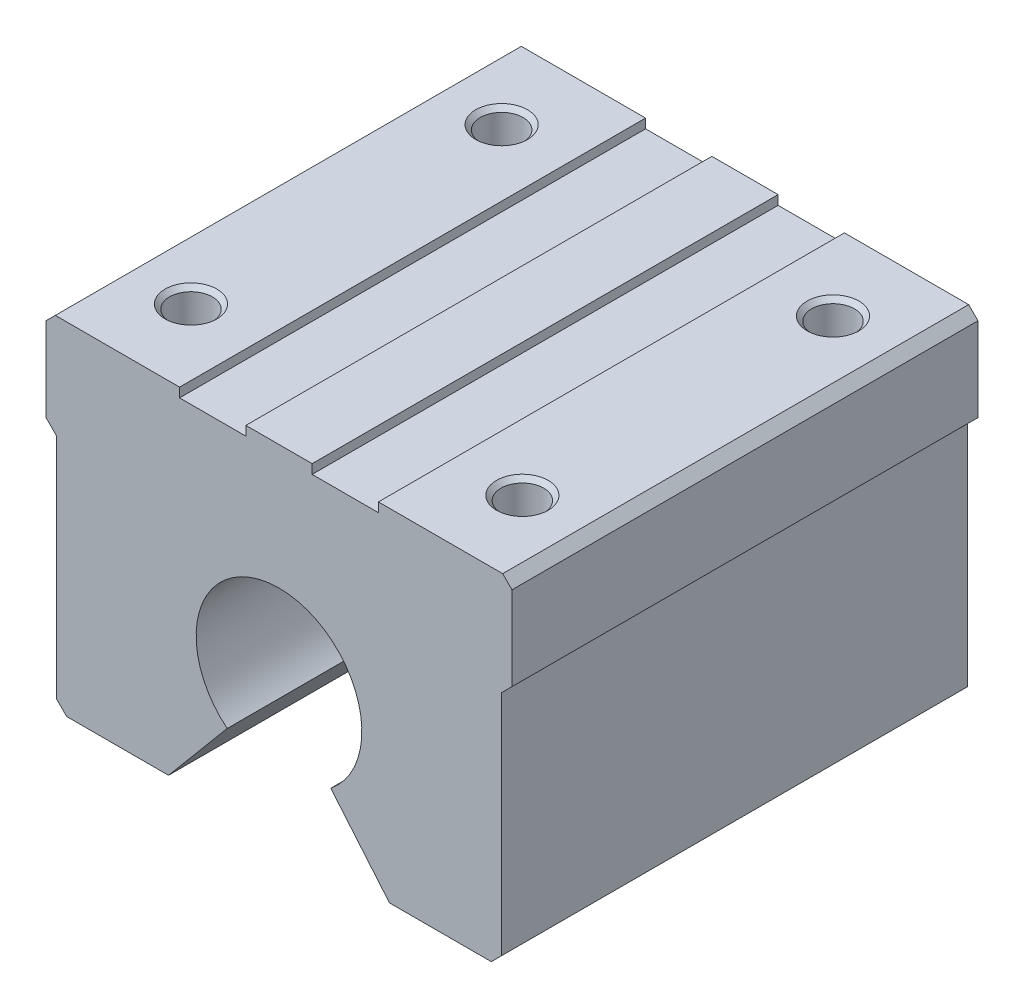
from build123d import *

# Parameters (mm, degrees)
SKETCH_1_W               = 45
SKETCH_1_H               = 45
EXTRUDE_1_DEPTH          = 33
SKETCH_2_W               = 6.4
SKETCH_2_H               = 0.9
CUT_EXTRUDE_1_DEPTH      = 68.5
SKETCH_3_W               = 6.4
SKETCH_3_H               = 0.9
CUT_EXTRUDE_2_DEPTH      = 68.5
SKETCH_4_W               = 1
SKETCH_4_H               = 24
CUT_EXTRUDE_3_DEPTH      = 68.5
CUT_EXTRUDE_4_DEPTH      = 68.5
SKETCH_6_W               = 1
SKETCH_6_H               = 24
CUT_EXTRUDE_5_DEPTH      = 68.500000167
DRAFT_1_ANGLE            = 45
DRAFT_2_ANGLE            = 45
DRAFT_3_ANGLE            = 40
HOLE_WIZARD_16_0_16_1_D  = 16.000000007
HOLE_WIZARD_M3_5_1_D     = 4.134
HOLE_WIZARD_M3_5_1_DEPTH = 15.60662
HOLE_WIZARD_M3_5_1_TIP   = 1.193383006
CHAMFER_1_SIZE           = 0.433
CHAMFER_2_SIZE           = 1
CHAMFER_3_SIZE           = 0.9
CUT_EXTRUDE_6_DEPTH      = 106.297198595


with BuildPart() as part:
    # 草图1 → 凸台-拉伸1 (new body)
    with BuildSketch(Plane.XZ.offset(-12)):
        with Locations((0, 230)):
            Rectangle(SKETCH_1_W, SKETCH_1_H)
    extrude(amount=-EXTRUDE_1_DEPTH)

    # 草图2 → 切除-拉伸1 (cut, through all)
    with BuildSketch(Plane.XY.offset(252.5)):
        with Locations((-6.4, 44.55)):
            Rectangle(SKETCH_2_W, SKETCH_2_H)
    extrude(amount=-CUT_EXTRUDE_1_DEPTH, mode=Mode.SUBTRACT)

    # 草图3 → 切除-拉伸2 (cut, through all)
    with BuildSketch(Plane.XY.offset(252.5)):
        with Locations((6.4, 44.55)):
            Rectangle(SKETCH_3_W, SKETCH_3_H)
    extrude(amount=-CUT_EXTRUDE_2_DEPTH, mode=Mode.SUBTRACT)

    # 草图4 → 切除-拉伸3 (cut, through all)
    with BuildSketch(Plane.XY.offset(252.5)):
        with Locations((22, 24)):
            Rectangle(SKETCH_4_W, SKETCH_4_H)
    extrude(amount=-CUT_EXTRUDE_3_DEPTH, mode=Mode.SUBTRACT)

    # 草图5 → 切除-拉伸4 (cut, through all)
    with BuildSketch(Plane.XY.offset(252.5)):
        with BuildLine():
            Line((-10.668119688, 12), (10.668119688, 12))
            add(Edge.make_bspline(
                [(5, 18.755002002), (6.889373229, 16.503334668), (8.778746459, 14.251667334), (10.668119688, 12)],
                knots=[0, 0, 0, 0, 1, 1, 1, 1], degree=3))
            Line((5, 18.755002002), (-10.668119688, 37.427539929))
            Line((-10.668119688, 37.427539929), (-10.668119688, 12))
        make_face()
    extrude(amount=-CUT_EXTRUDE_4_DEPTH, mode=Mode.SUBTRACT)

    # 草图6 → 切除-拉伸5 (cut, through all)
    with BuildSketch(Plane.XY.offset(252.5)):
        with Locations((-22, 24)):
            Rectangle(SKETCH_6_W, SKETCH_6_H)
    extrude(amount=-CUT_EXTRUDE_5_DEPTH, mode=Mode.SUBTRACT)

    # 拔模1
    draft_1_faces = [part.faces().sort_by_distance(p)[0] for p in [
        (-22, 36, 230),
    ]]
    draft(draft_1_faces, Plane(origin=(-22.5, 45, 252.5), x_dir=(0, 0, -1), z_dir=(-1, 0, 0)), DRAFT_1_ANGLE)

    # 拔模2
    draft_2_faces = [part.faces().sort_by_distance(p)[0] for p in [
        (22, 36, 230),
    ]]
    draft(draft_2_faces, Plane(origin=(22.5, 45, 207.5), x_dir=(0, 0, 1), z_dir=(1, 0, 0)), DRAFT_2_ANGLE)

    # 拔模3
    draft_3_faces = [part.faces().sort_by_distance(p)[0] for p in [
        (-10.668119688, 24.713769965, 230),
    ]]
    draft(draft_3_faces, Plane(origin=(0, 12, 0), x_dir=(0, 0, -1), z_dir=(0, -1, 0)), DRAFT_3_ANGLE)

    # Ø16.0 (16) 直径孔1 (through all)
    with Locations(Plane(origin=(0, 0, 207.5), x_dir=(-1, 0, 0), z_dir=(0, 0, -1))):
        with Locations((0, 25)):
            Hole(HOLE_WIZARD_16_0_16_1_D / 2)

    # M3.5 间隙孔1
    with Locations(Plane(origin=(0, 45, 0), x_dir=(1, 0, 0), z_dir=(0, 1, 0))):
        with Locations((16, -215), (16, -245), (-16, -215), (-16, -245)):
            Hole(HOLE_WIZARD_M3_5_1_D / 2, depth=HOLE_WIZARD_M3_5_1_DEPTH)
            with Locations((0, 0, -(HOLE_WIZARD_M3_5_1_DEPTH + HOLE_WIZARD_M3_5_1_TIP / 2))):  # 120° drill point
                Cone(0, HOLE_WIZARD_M3_5_1_D / 2, HOLE_WIZARD_M3_5_1_TIP, mode=Mode.SUBTRACT)

    # 倒角1
    chamfer_1_edges = [part.edges().sort_by_distance(p)[0] for p in [
        (-13.933, 45, 245),
        (-13.933, 45, 215),
        (18.067, 45, 245),
        (18.067, 45, 215),
    ]]
    chamfer(chamfer_1_edges, length=CHAMFER_1_SIZE)

    # 倒角2
    chamfer_2_edges = [part.edges().sort_by_distance(p)[0] for p in [
        (21.5, 12, 230),
        (-21.5, 12, 230),
    ]]
    chamfer(chamfer_2_edges, length=CHAMFER_2_SIZE)

    # 倒角3
    chamfer_3_edges = [part.edges().sort_by_distance(p)[0] for p in [
        (-22.5, 45, 230),
        (22.5, 45, 230),
    ]]
    chamfer(chamfer_3_edges, length=CHAMFER_3_SIZE)

    # 草图11 → 切除-拉伸6 (cut, through all)
    with BuildSketch(Plane.XY.offset(300)):
        with BuildLine():
            Line((-9.25, 11.7), (-9.25, 5))
            Line((-9.25, 5), (-20, 5))
            Line((-20, 5), (-20, 0))
            Line((-20, 0), (20, 0))
            Line((20, 0), (20, 5))
            Line((20, 5), (9.25, 5))
            Line((9.25, 5), (9.25, 11.7))
            Line((9.25, 11.7), (9.11850775, 11.7))
            Line((9.11850775, 11.7), (4, 17.8))
            Line((4, 17.8), (3.487119155, 17.8))
            ThreePointArc((3.487119155, 17.8), (0, 33), (-3.487119155, 17.8))
            Line((-3.487119155, 17.8), (-4, 17.8))
            Line((-4, 17.8), (-9.11850775, 11.7))
            Line((-9.11850775, 11.7), (-9.25, 11.7))
        make_face()
    extrude(amount=-CUT_EXTRUDE_6_DEPTH, mode=Mode.SUBTRACT)


solid = part.part
